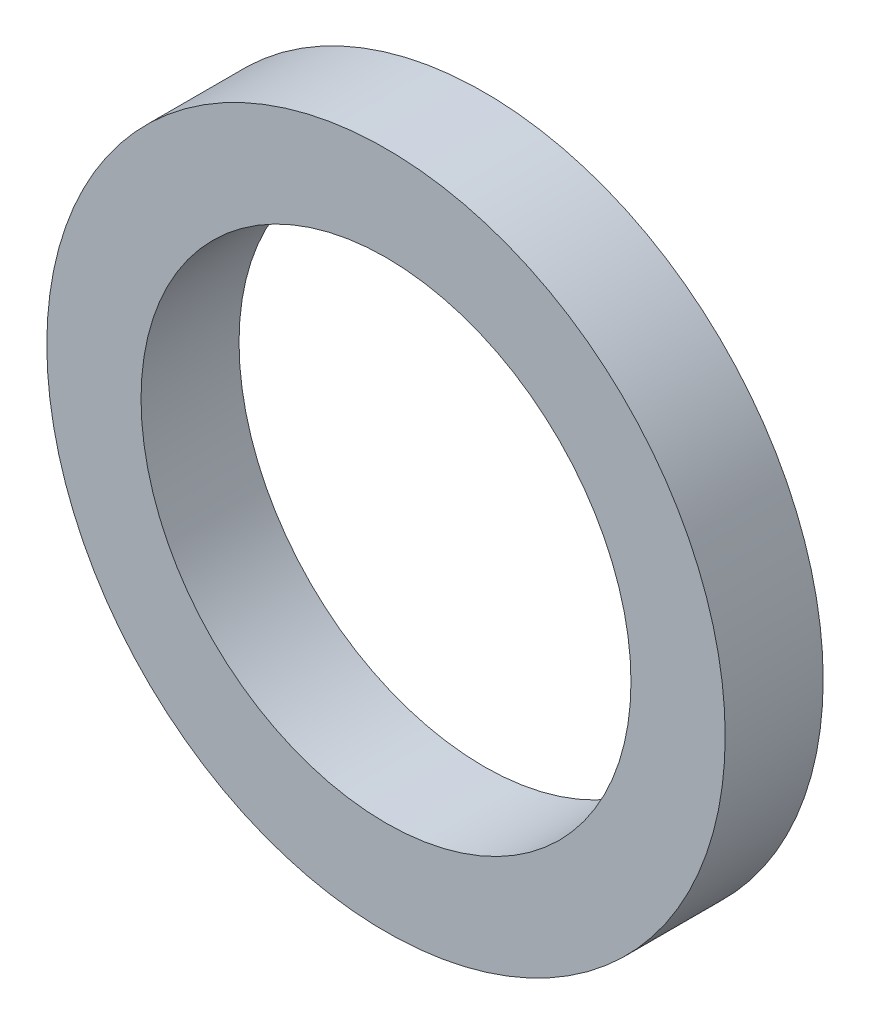
SolidWorks part; units mm, degrees
ref_plane "Front Plane" through (0, 0, 0) normal (0, 0, 1) x (1, 0, 0)
ref_plane "Top Plane" through (0, 0, 0) normal (0, 1, 0) x (1, 0, 0)
ref_plane "Right Plane" through (0, 0, 0) normal (1, 0, 0) x (0, 0, -1)
sketch "Sketch1" plane through (0, 0, 0) normal (0, 0, 1) x (1, 0, 0)
  circle A0 centre (0, 0) radius 65
  circle A1 centre (0, 0) radius 90
  dimension "D1" = 180
  dimension "D2" = 130
extrude "Boss-Extrude1" add sketch "Sketch1" along normal blind 26
